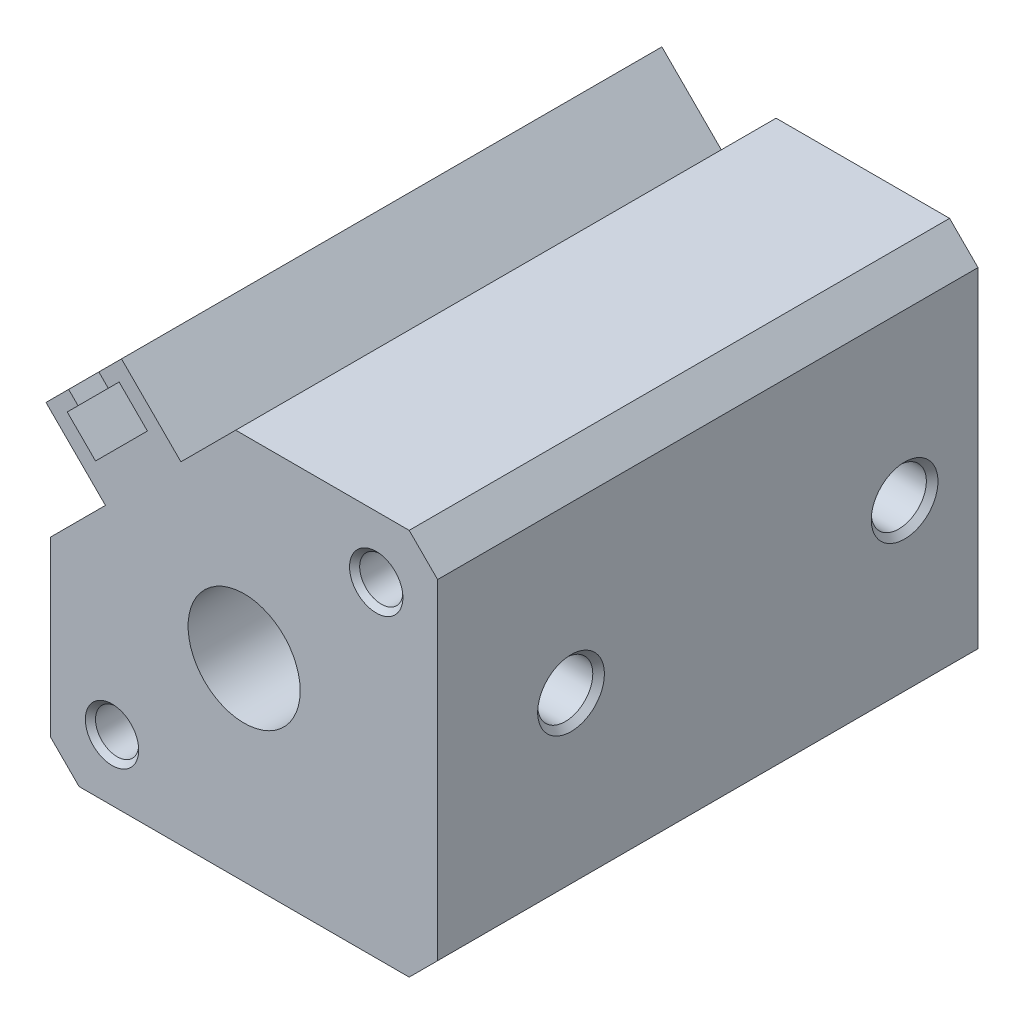
SolidWorks part; units mm, degrees
ref_plane "前视" through (0, 0, 0) normal (0, 0, 1) x (1, 0, 0)
ref_plane "上视" through (0, 0, 0) normal (0, 1, 0) x (1, 0, 0)
ref_plane "右视" through (0, 0, 0) normal (1, 0, 0) x (0, 0, -1)
sketch "草图1" plane through (0, 0, 0) normal (0, 0, 1) x (1, 0, 0)
  line L0 (-14.8492, 9.1924) -> (-10.3945, 4.7376)
  line L1 (-10.3945, 4.7376) -> (-14.5, 0.6321)
  line L2 (-14.5, 0.6321) -> (-14.5, -12.3701)
  line L3 (-14.5, -12.3701) -> (-12.3701, -14.5)
  line L4 (-12.3701, -14.5) -> (12.3701, -14.5)
  line L5 (12.3701, -14.5) -> (14.5, -12.3701)
  line L6 (14.5, -12.3701) -> (14.5, 12.3701)
  line L7 (14.5, 12.3701) -> (12.3701, 14.5)
  line L8 (12.3701, 14.5) -> (-0.6321, 14.5)
  line L9 (-0.6321, 14.5) -> (-4.7376, 10.3945)
  line L10 (-4.7376, 10.3945) -> (-9.1924, 14.8492)
  line L11 (-9.1924, 14.8492) -> (-10.8894, 13.1522)
  line L12 (-10.8894, 13.1522) -> (-10.1823, 12.4451)
  line L13 (-10.1823, 12.4451) -> (-9.3692, 13.2583)
  line L14 (-9.3692, 13.2583) -> (-7.2478, 11.1369)
  line L15 (-7.2478, 11.1369) -> (-11.1369, 7.2478)
  line L16 (-11.1369, 7.2478) -> (-13.2583, 9.3692)
  line L17 (-13.2583, 9.3692) -> (-12.4451, 10.1823)
  line L18 (-12.4451, 10.1823) -> (-13.1522, 10.8894)
  line L19 (-13.1522, 10.8894) -> (-14.8492, 9.1924)
extrude "凸台-拉伸1" add sketch "草图1" against normal blind 40.5
sketch "草图2" plane through (0, 0, 0) normal (0, 1, 0) x (1, 0, 0)
  line L0 (8.5, 10) -> (8.5, 12.065)
  line L1 (8.5, 12.065) -> (14.065, 12.065)
  line L2 (14.065, 12.065) -> (15, 13)
  line L3 (15, 13) -> (15, 10)
  line L4 (15, 10) -> (8.5, 10)
  line L5 (15, 10) -> (8.5, 10) construction
revolve "切除-旋转1" cut sketch "草图2" angle 360 about L5
sketch "草图3" plane through (0, 0, 0) normal (0, 1, 0) x (1, 0, 0)
  line L0 (8.5, 35) -> (8.5, 37.065)
  line L1 (8.5, 37.065) -> (14.065, 37.065)
  line L2 (14.065, 37.065) -> (15, 38)
  line L3 (15, 38) -> (15, 35)
  line L4 (15, 35) -> (8.5, 35)
  line L5 (15, 35) -> (8.5, 35) construction
revolve "切除-旋转2" cut sketch "草图3" angle 360 about L5
ref_plane "基准面1" through (0, 0, 0) normal (0.7071, -0.7071, 0) x (-0.7071, -0.7071, 0)
sketch "草图4" plane through (0, 0, 0) normal (0.7071, -0.7071, 0) x (-0.7071, -0.7071, 0)
  line L0 (-14, -0.5) -> (-16.5, -0.5)
  line L1 (-16.5, -0.5) -> (-15.62, 0.38)
  line L2 (-15.62, 0.38) -> (-15.62, 40.12)
  line L3 (-15.62, 40.12) -> (-16.5, 41)
  line L4 (-16.5, 41) -> (-14, 41)
  line L5 (-14, 41) -> (-14, -0.5)
  line L6 (-14, 41) -> (-14, -0.5) construction
revolve "切除-旋转3" cut sketch "草图4" angle 360 about L6
sketch "草图5" plane through (0, 0, 0) normal (0.7071, -0.7071, 0) x (-0.7071, -0.7071, 0)
  line L0 (14, -0.5) -> (11.5, -0.5)
  line L1 (11.5, -0.5) -> (12.38, 0.38)
  line L2 (12.38, 0.38) -> (12.38, 40.12)
  line L3 (12.38, 40.12) -> (11.5, 41)
  line L4 (11.5, 41) -> (14, 41)
  line L5 (14, 41) -> (14, -0.5)
  line L6 (14, 41) -> (14, -0.5) construction
revolve "切除-旋转4" cut sketch "草图5" angle 360 about L6
ref_plane "基准面2" through (0, 14, 0) normal (0, 1, 0) x (1, 0, 0)
ref_plane "基准面3" through (0, -14, 0) normal (0, 1, 0) x (1, 0, 0)
ref_plane "基准面4" through (0, 0, -40.5) normal (0, 0, 1) x (1, 0, 0)
ref_plane "基准面5" through (0, 0, 0) normal (0, 0, 1) x (1, 0, 0)
ref_plane "基准面6" through (0, 0, -40.5) normal (0, 0, 1) x (1, 0, 0)
ref_plane "基准面7" through (0, -19, 0) normal (0, 1, 0) x (1, 0, 0)
ref_plane "基准面8" through (0, 0, 0) normal (0, 0, 1) x (1, 0, 0)
ref_plane "基准面9" through (0, 0, -40.5) normal (0, 0, 1) x (1, 0, 0)
ref_plane "基准面10" through (0, 0, 2) normal (0, 0, 1) x (1, 0, 0)
ref_plane "基准面11" through (0, 0, -42.5) normal (0, 0, 1) x (1, 0, 0)
ref_plane "基准面12" through (0, 0, -40.5) normal (0, 0, 1) x (1, 0, 0)
ref_plane "基准面13" through (0, 0, -44.5) normal (0, 0, 1) x (1, 0, 0)
ref_plane "基准面14" through (0, 0, -44.5) normal (0, 0, 1) x (1, 0, 0)
ref_plane "基准面15" through (0, 0, -45.5) normal (0, 0, 1) x (1, 0, 0)
ref_plane "基准面16" through (0, 0, 0) normal (0, 0, 1) x (1, 0, 0)
ref_plane "基准面17" through (0, 0, -40.5) normal (0, 0, 1) x (1, 0, 0)
ref_plane "基准面18" through (0, -19, 0) normal (0, 1, 0) x (1, 0, 0)
ref_plane "基准面19" through (0, 0, 2) normal (0, 0, 1) x (1, 0, 0)
ref_plane "基准面20" through (0, 0, -42.5) normal (0, 0, 1) x (1, 0, 0)
ref_plane "基准面21" through (0, 0, -40.5) normal (0, 0, 1) x (1, 0, 0)
ref_plane "基准面22" through (0, 0, -44.5) normal (0, 0, 1) x (1, 0, 0)
ref_plane "基准面23" through (-3.25, 0, 0) normal (1, 0, 0) x (0, 0, -1)
ref_plane "基准面24" through (3.25, 0, 0) normal (1, 0, 0) x (0, 0, -1)
ref_plane "基准面25" through (0, 0, -44.5) normal (0, 0, 1) x (1, 0, 0)
ref_plane "基准面26" through (0, 0, -1) normal (0, 0, 1) x (1, 0, 0)
ref_plane "基准面27" through (0, 0, -39.5) normal (0, 0, 1) x (1, 0, 0)
ref_plane "基准面28" through (0, 0, -1) normal (0, 0, 1) x (1, 0, 0)
ref_plane "基准面29" through (0, 0, -39.5) normal (0, 0, 1) x (1, 0, 0)
ref_plane "基准面30" through (0, 0, -1) normal (0, 0, 1) x (1, 0, 0)
sketch "草图6" plane through (0, 0, 0) normal (0, 0, 1) x (1, 0, 0)
  circle A0 centre (0, 0) radius 4.2
extrude "切除-拉伸1" cut sketch "草图6" against normal blind 20
